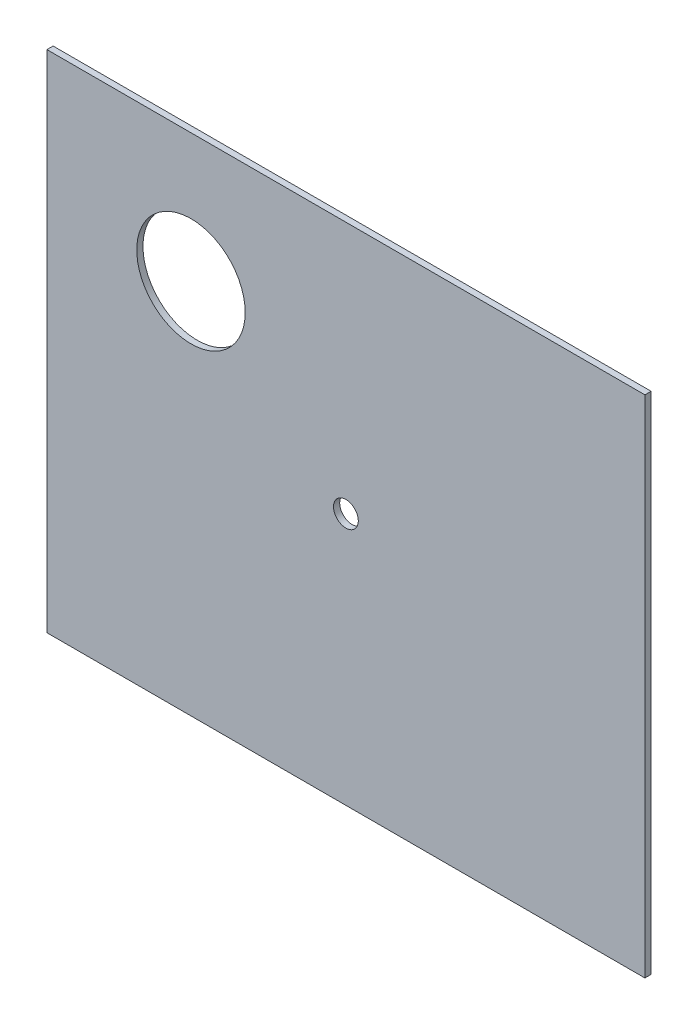
SolidWorks part; units mm, degrees
ref_plane "前视基准面" through (0, 0, 0) normal (0, 0, 1) x (1, 0, 0)
ref_plane "上视基准面" through (0, 0, 0) normal (0, 1, 0) x (1, 0, 0)
ref_plane "右视基准面" through (0, 0, 0) normal (1, 0, 0) x (0, 0, -1)
other "Configuration Table"
sketch "草图1" plane through (0, 0, 0) normal (0, 0, 1) x (1, 0, 0)
  line L0 (-193, -163) -> (193, -163)
  line L1 (193, -163) -> (193, 163)
  line L2 (193, 163) -> (-193, 163)
  line L3 (-193, 163) -> (-193, -163)
  point P0 (0, 0)
  dimension "D1" = 193
  dimension "D2" = 386
  dimension "D3" = 163
  dimension "D4" = 326
extrude "凸台-拉伸1" add sketch "草图1" against normal mid plane 4
sketch "草图2" plane through (0, 0, 0) normal (0, 0, 1) x (1, 0, 0)
  circle A0 centre (0, 0) radius 8
  circle A1 centre (-100, 80) radius 35
  point P0 (0, 0)
  dimension "D1" = 16
  dimension "D2" = 70
  dimension "D3" = 100
  dimension "D4" = 80
extrude "切除-拉伸1" cut sketch "草图2" against normal mid plane 24
